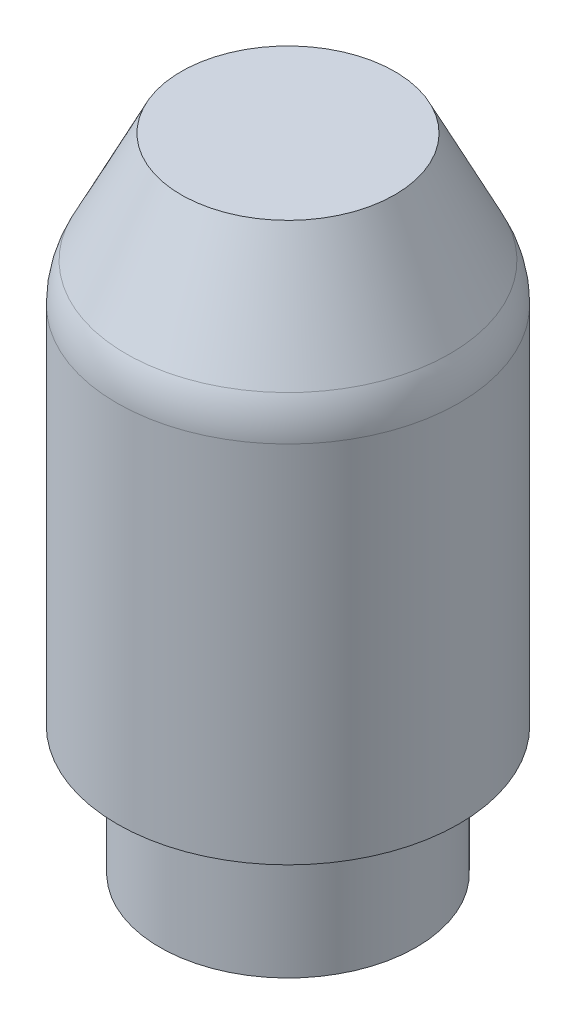
from build123d import *

# Parameters (mm, degrees)
M3_TAPPED_HOLE1_D     = 2.5
M3_TAPPED_HOLE1_DEPTH = 10
M3_TAPPED_HOLE1_TIP   = 0.751075774
FILLET1_R             = 2


with BuildPart() as part:
    # Sketch1 → Revolve1 (revolve)
    with BuildSketch(Plane.XY):
        Polygon((0, 0), (0, 15), (2.5, 15), (4, 12), (4, 3), (3, 3), (3, 0), align=None)
    revolve(axis=Axis((0, 0, 0), (0, 1, 0)))

    # M3 Tapped Hole1
    with Locations(Plane(origin=(0, 0, 0), x_dir=(-1, 0, 0), z_dir=(0, -1, 0))):
        with Locations((0, 0)):
            Hole(M3_TAPPED_HOLE1_D / 2, depth=M3_TAPPED_HOLE1_DEPTH)
            with Locations((0, 0, -(M3_TAPPED_HOLE1_DEPTH + M3_TAPPED_HOLE1_TIP / 2))):  # 118° drill point
                Cone(0, M3_TAPPED_HOLE1_D / 2, M3_TAPPED_HOLE1_TIP, mode=Mode.SUBTRACT)

    # Fillet1
    fillet1_edges = [part.edges().sort_by_distance(p)[0] for p in [
        (-4, 12, 0),
    ]]
    fillet(fillet1_edges, radius=FILLET1_R)


solid = part.part
